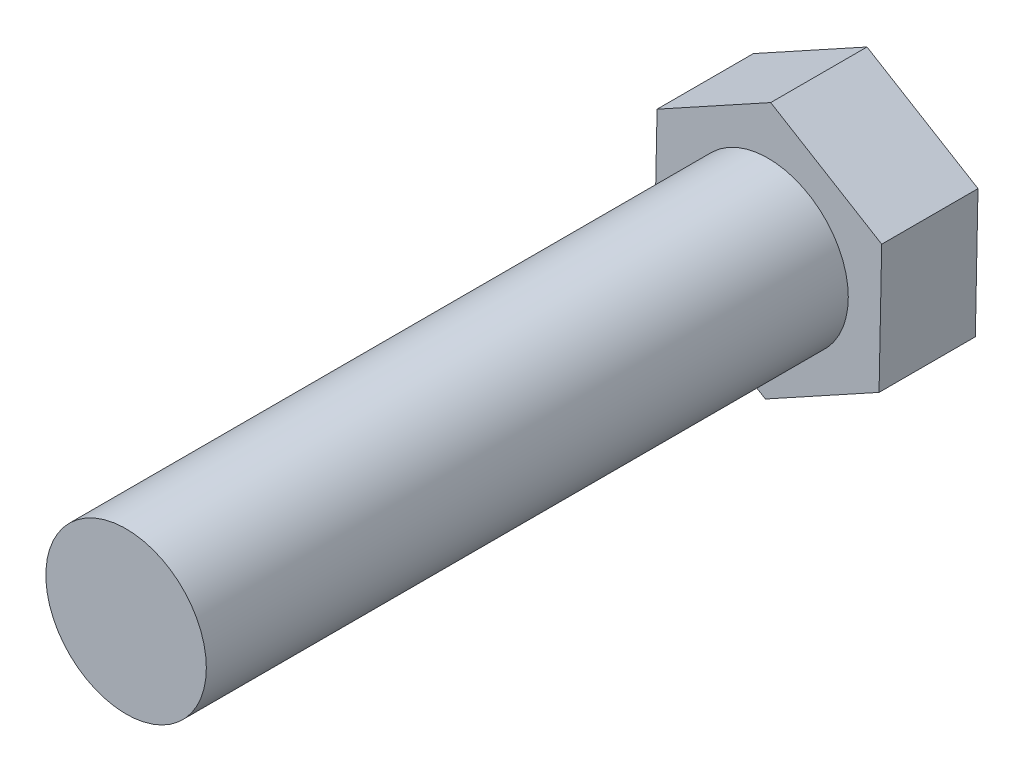
from build123d import *

# Parameters (mm, degrees)
SKETCH_1_R      = 2.5
EXTRUDE_1_DEPTH = 20
EXTRUDE_2_DEPTH = 3


with BuildPart() as part:
    # 草图1 → 凸台-拉伸1 (new body)
    with BuildSketch(Plane.XY):
        Circle(SKETCH_1_R)
    extrude(amount=EXTRUDE_1_DEPTH)

    # 草图2 → 凸台-拉伸2 (add)
    with BuildSketch(Plane(origin=(0, 0, 0), x_dir=(-1, 0, 0), z_dir=(0, 0, -1))):
        Polygon((0.082884141, -4.04060188), (3.540705945, -1.948521168), (3.457821804, 2.092080712), (-0.082884141, 4.04060188), (-3.540705945, 1.948521168), (-3.457821804, -2.092080712), align=None)
    extrude(amount=EXTRUDE_2_DEPTH)


solid = part.part
